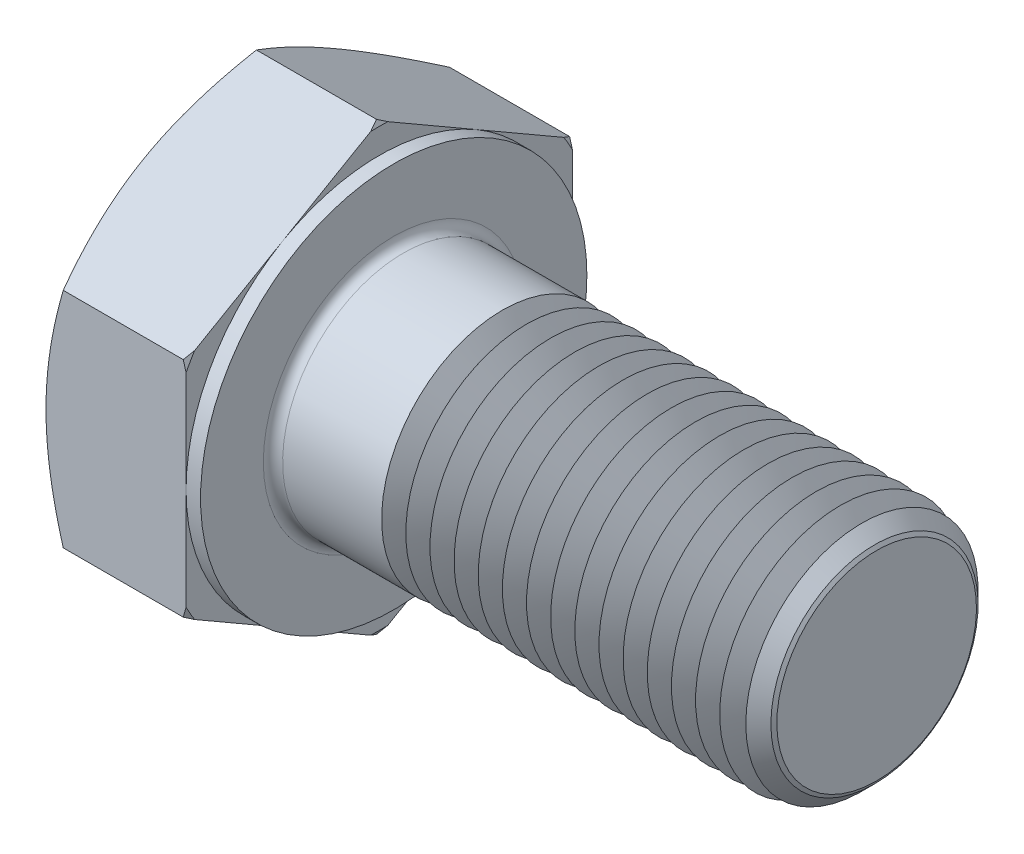
from build123d import *

# Parameters (mm, degrees)
EXTRUDE_393_DEPTH      = 6.4
SKETCH_4_W             = 0.6
SKETCH_4_H             = 11.237604307
CHAMFER_2075_SIZE      = 0.8
FILLET_2120_R          = 0.4
PATTERN_LINEAR_1_COUNT = 16
PATTERN_LINEAR_1_PITCH = 1


with BuildPart() as part:
    # 草图1 → Extrude 393 (new body)
    with BuildSketch(Plane(origin=(0, 0, 0), x_dir=(0, 0, -1), z_dir=(1, 0, 0))):
        Polygon((8, 4.618802154), (8, -4.618802154), (0, -9.237604307), (-8, -4.618802154), (-8, 4.618802154), (0, 9.237604307), align=None)
    extrude(amount=EXTRUDE_393_DEPTH)

    # 草图2 → 凸台-旋转1 (revolve)
    with BuildSketch(Plane.XY, mode=Mode.PRIVATE) as revolve_1_sk:
        Polygon((0, 0), (26.4, 0), (26.4, 4.134), (26.4, 5), (0, 5), align=None)
    revolve(revolve_1_sk.sketch.rotate(Axis((0, 0, 0), (1, 0, 0)), 90), axis=Axis((0, 0, 0), (1, 0, 0)))

    # 草图3 → 切除-旋转1 (revolve, cut)
    with BuildSketch(Plane.XY):
        Polygon((0, 8), (3.601282526, 14.237604307), (3.601282526, 19.237604307), (-10, 19.237604307), (-10, 8), align=None)
    revolve(axis=Axis((0, 0, 0), (1, 0, 0)), mode=Mode.SUBTRACT)

    # 草图5 → 切除-旋转2 (revolve, cut)
    with BuildSketch(Plane.XY):
        Polygon((6.4, 8), (2.798717474, 14.237604307), (2.798717474, 19.237604307), (12.798717474, 19.237604307), (12.798717474, 8), align=None)
    revolve(axis=Axis((0, 0, 0), (1, 0, 0)), mode=Mode.SUBTRACT)

    # 草图4 → 切除-旋转3 (revolve, cut)
    with BuildSketch(Plane.XY, mode=Mode.PRIVATE) as cut_revolve_3_sk:
        with Locations((6.1, 13.618802154)):
            Rectangle(SKETCH_4_W, SKETCH_4_H)
    revolve(cut_revolve_3_sk.sketch.rotate(Axis((0, 0, 0), (1, 0, 0)), 270), axis=Axis((0, 0, 0), (1, 0, 0)), mode=Mode.SUBTRACT)

    # Chamfer 2075
    chamfer_2075_edges = [part.edges().sort_by_distance(p)[0] for p in [
        (26.4, 0, -5),
    ]]
    chamfer(chamfer_2075_edges, length=CHAMFER_2075_SIZE)

    # Fillet 2120
    fillet_2120_edges = [part.edges().sort_by_distance(p)[0] for p in [
        (6.4, 0, -5),
    ]]
    fillet(fillet_2120_edges, radius=FILLET_2120_R)

    # 草图6 → 切除-旋转4 (revolve, cut)
    with BuildSketch(Plane.XY):
        Polygon((11.4, -4.134), (10.900014667, -5), (10.900014667, -6.25), (11.899985333, -6.25), (11.899985333, -5), align=None)
    cut_revolve_4 = revolve(axis=Axis((-3.175, 0, 0), (1, 0, 0)), mode=Mode.SUBTRACT)

    # 阵列(线性)1: 切除-旋转4 ×16
    with Locations(*[(i * PATTERN_LINEAR_1_PITCH, 0, 0) for i in range(1, PATTERN_LINEAR_1_COUNT)]):
        add(cut_revolve_4, mode=Mode.SUBTRACT)


solid = part.part
